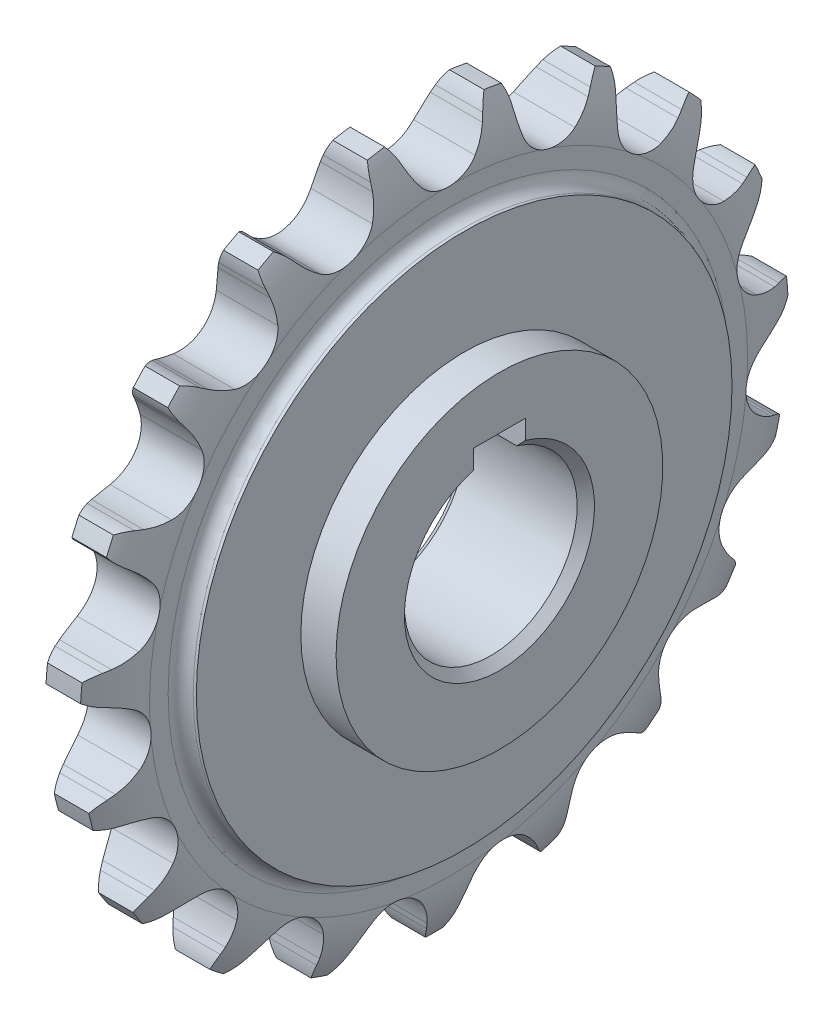
SolidWorks part; units mm, degrees
ref_plane "前视基准面" through (0, 0, 0) normal (0, 0, 1) x (1, 0, 0)
ref_plane "上视基准面" through (0, 0, 0) normal (0, 1, 0) x (1, 0, 0)
ref_plane "右视基准面" through (0, 0, 0) normal (1, 0, 0) x (0, 0, -1)
sketch "草图1" plane through (0, 0, 0) normal (0, 0, 1) x (1, 0, 0)
  line L0 (-6.35, 0) -> (6.35, 0) construction
  line L1 (-5.4601, 10) -> (-5.4601, 31)
  line L2 (-5.4601, 31) -> (-5.0981, 31)
  line L3 (-3.6502, 32.4479) -> (-3.6502, 34.6196)
  line L4 (-1.9992, 41) -> (1.9992, 41)
  line L5 (3.6502, 34.6196) -> (3.6502, 32.4479)
  line L6 (5.0981, 31) -> (5.4601, 31)
  line L7 (5.4601, 31) -> (5.4601, 10)
  line L8 (5.4601, 10) -> (-5.4601, 10)
  line L9 (0, 0) -> (0, 41) construction
  line L10 (-3.0556, 38.5796) -> (3.0556, 38.5796) construction
  line L11 (-3.0556, -38.5796) -> (3.0556, -38.5796) construction
  line L12 (6.35, 0) -> (25.35, 0) construction
  line L13 (-3.6502, 34.6196) -> (3.7984, 34.6196) construction
  line L14 (-3.6502, -34.6196) -> (3.7984, -34.6196) construction
  line L15 (25.35, 0) -> (33.27, 0) construction
  line L16 (33.27, 0) -> (45.34, 0) construction
  line L17 (45.34, 0) -> (53.19, 0) construction
  line L18 (53.19, 0) -> (67.57, 0) construction
  arc A0 (-1.9992, 41) -> (-3.6502, 34.6196) centre (9.0492, 34.7373) ccw
  arc A1 (1.9992, 41) -> (3.6502, 34.6196) centre (-9.0492, 34.7373) cw
  arc A2 (3.6502, 32.4479) -> (5.0981, 31) centre (5.0981, 32.4479) ccw
  arc A3 (-5.0981, 31) -> (-3.6502, 32.4479) centre (-5.0981, 32.4479) ccw
  point P30 (3.6502, 31)
  point P33 (-3.6502, 31)
  dimension "D1" = 3.6196
  dimension "rx" = 12.7
  dimension "D3" = 1.4479
  dimension "d" = 77.1593
  dimension "p" = 12.7
  dimension "z" = 19
  dimension "da" = 82
  dimension "df" = 69.2393
  dimension "dr" = 7.92
  dimension "dk" = 20
  dimension "dg" = 62
  dimension "h" = 12.07
  dimension "bf1" = 7.3005
  dimension "b1" = 7.85
  dimension "ba" = 1.651
  dimension "D2" = 1.8098
  dimension "pt" = 14.38
revolve "旋转1" add sketch "草图1" angle 360 about L0
sketch "草图2" plane through (0, 0, 0) normal (1, 0, 0) x (0, 0, -1)
  line L0 (0, 0) -> (0, 41) construction
  line L1 (0, 0) -> (-6.7484, 40.4408) construction
  line L2 (0, 0) -> (-13.3127, 38.7785) construction
  line L3 (3.1687, 36.0899) -> (3.1879, 36.0748) construction
  line L4 (4.5522, 38.4265) -> (-4.9821, 42.4942) construction
  line L5 (0, 0) -> (6.7484, 40.4408) construction
  line L6 (4.5522, 38.4265) -> (4.8587, 39.1448)
  line L7 (-4.5522, 38.4265) -> (-4.8587, 39.1448)
  circle A0 centre (0, 0) radius 41 construction
  arc A1 (3.1687, 36.0899) -> (-3.1687, 36.0899) centre (0, 38.5796) cw
  arc A2 (3.1687, 36.0899) -> (4.5522, 38.4265) centre (-4.9821, 42.4942) ccw
  arc A3 (5.7509, 40.5947) -> (4.8587, 39.1448) centre (10.1556, 36.885) ccw
  arc A4 (-3.1687, 36.0899) -> (-4.5522, 38.4265) centre (4.9821, 42.4942) cw
  arc A5 (-5.7509, 40.5947) -> (-4.8587, 39.1448) centre (-10.1556, 36.885) cw
  arc A7 (5.7509, 40.5947) -> (-5.7509, 40.5947) centre (0, 0) ccw
  dimension "r1" = 4.0298
  dimension "r3" = 5.7588
  dimension "D1" = 18.947
  dimension "D2" = 9.474
  dimension "α/2" = 51.842
  dimension "M" = 4.9821
  dimension "T" = 3.9146
  dimension "β" = 15.053
  dimension "γ/2" = 13.632
  dimension "bc" = 0.781
extrude "切除-拉伸1" cut sketch "草图2" against normal mid plane 10.9201
pattern_circular "阵列(圆周)1" count 19 over 360 about axis through (0, 0, 0) along (1, 0, 0) of "切除-拉伸1"
sketch "草图3" plane through (0, 0, 0) normal (0, 0, 1) x (1, 0, 0)
  line L0 (5.4601, 10) -> (9.5399, 10)
  line L3 (9.5399, 10) -> (9.5399, 18.9049)
  line L4 (9.5399, 18.9049) -> (5.4601, 18.9049)
  line L5 (5.4601, 18.9049) -> (5.4601, 10)
  line L6 (0, 0) -> (4.8, 0) construction
  line L8 (-5.4601, 31) -> (-5.4601, -31) construction
  dimension "h" = 8.9049
  dimension "K" = 4.8
  dimension "L" = 15
revolve "旋转2" add sketch "草图3" angle 360 about L6
sketch "草图4" plane through (-5.4601, 0, 0) normal (-1, 0, 0) x (0, 0, 1)
  line L1 (-3, 9.5394) -> (3, 9.5394)
  line L2 (-3, 9.5394) -> (-3, 12.8)
  line L3 (-3, 12.8) -> (3, 12.8)
  line L4 (3, 9.5394) -> (3, 12.8)
  circle A0 centre (0, 0) radius 10 construction
  point P6 (0.2, 12.8)
  dimension "D1" = 12.8
  dimension "键槽宽度" = 6
  dimension "t1" = 2.8
extrude "切除-拉伸2" cut sketch "草图4" against normal through all
chamfer "倒角1" distance 1 angle 45 1 edges at (-5.4601, -10, 0)
chamfer "倒角3" distance 1 angle 45 1 edges at (9.5399, -10, 0)
